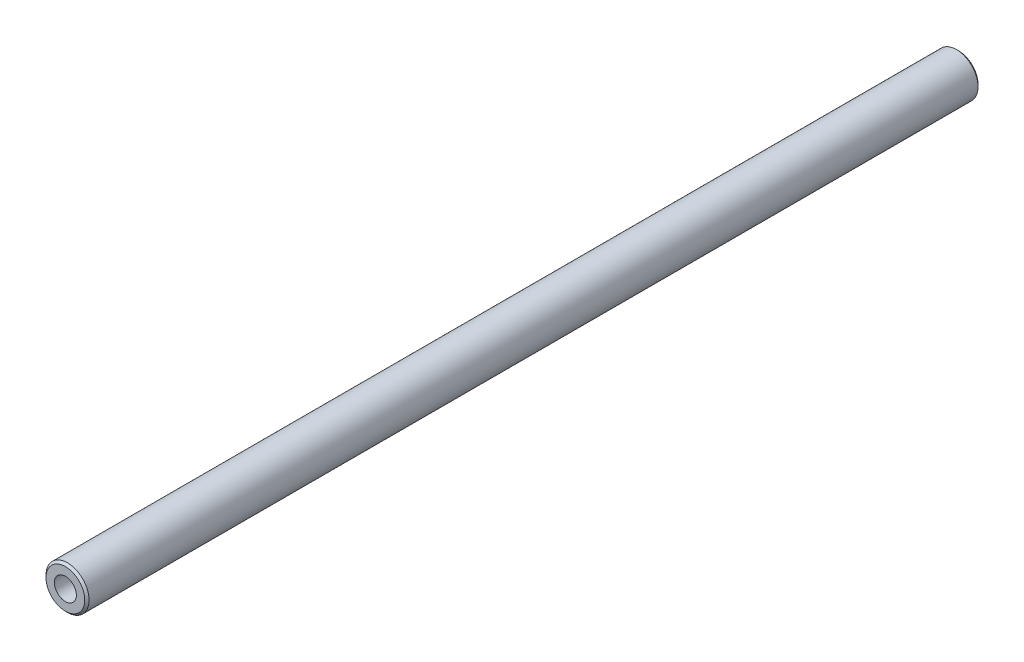
SolidWorks part; units mm, degrees
material "1023 碳钢板 (SS)"
ref_plane "前视基准面" through (0, 0, 0) normal (0, 0, 1) x (1, 0, 0)
ref_plane "上视基准面" through (0, 0, 0) normal (0, 1, 0) x (1, 0, 0)
ref_plane "右视基准面" through (0, 0, 0) normal (1, 0, 0) x (0, 0, -1)
ref_plane "基准面4" through (0, 0, 0) normal (0, -1, 0) x (1, 0, 0)
sketch "草图1" plane through (0, 0, 0) normal (0, -1, 0) x (1, 0, 0)
  line L6 (9, -207.5) -> (10, -206.5)
  line L7 (10, -206.5) -> (10, 206.5)
  line L8 (10, 206.5) -> (9, 207.5)
  line L10 (0, 207.5) -> (0, -207.5) construction
  line L13 (9, 207.5) -> (0, 207.5)
  line L14 (0, 207.5) -> (0, -207.5)
  line L15 (0, -207.5) -> (9, -207.5)
revolve "旋转1" add sketch "草图1" angle 360 about L10
hole_wizard "M12 螺纹孔5" positions "草图13" profile "草图9" tap size "M12" standard "GB"
sketch "草图13" plane through (0, 0, -207.5) normal (0, 0, -1) x (-1, 0, 0)
  point P0 (0, 0)
sketch "草图9" plane through (0, 0, -207.5) normal (1, 0, 0) x (0, 1, 0)
  line L0 (0, 0) -> (0, 223.0644)
  line L1 (0, 223.0644) -> (5.1, 220)
  line L2 (5.1, 220) -> (5.1, 0)
  line L5 (5.1, 0) -> (0, 0)
  line L10 (0, 223.0644) -> (-5.1, 220) construction
  line L11 (0, -6.35) -> (0, 107.95) construction
  dimension "螺纹孔钻头直径" = 10.2
  dimension "螺纹孔钻头深度" = 220
  dimension "导头角度" = 118
cosmetic thread "孔螺蚊线5"
hole_wizard "M12 螺纹孔6" positions "草图14" profile "草图15" tap size "M12" standard "GB"
sketch "草图14" plane through (0, 0, 207.5) normal (0, 0, 1) x (1, 0, 0)
  point P0 (0, 0)
sketch "草图15" plane through (0, 0, 207.5) normal (1, 0, 0) x (0, -1, 0)
  line L0 (0, 0) -> (0, 223.0644)
  line L1 (0, 223.0644) -> (5.1, 220)
  line L2 (5.1, 220) -> (5.1, 0)
  line L5 (5.1, 0) -> (0, 0)
  line L10 (0, 223.0644) -> (-5.1, 220) construction
  line L11 (0, -6.35) -> (0, 107.95) construction
  dimension "螺纹孔钻头直径" = 10.2
  dimension "螺纹孔钻头深度" = 220
  dimension "导头角度" = 118
cosmetic thread "孔螺蚊线6" parameters "D1"=40, "D2"=12
